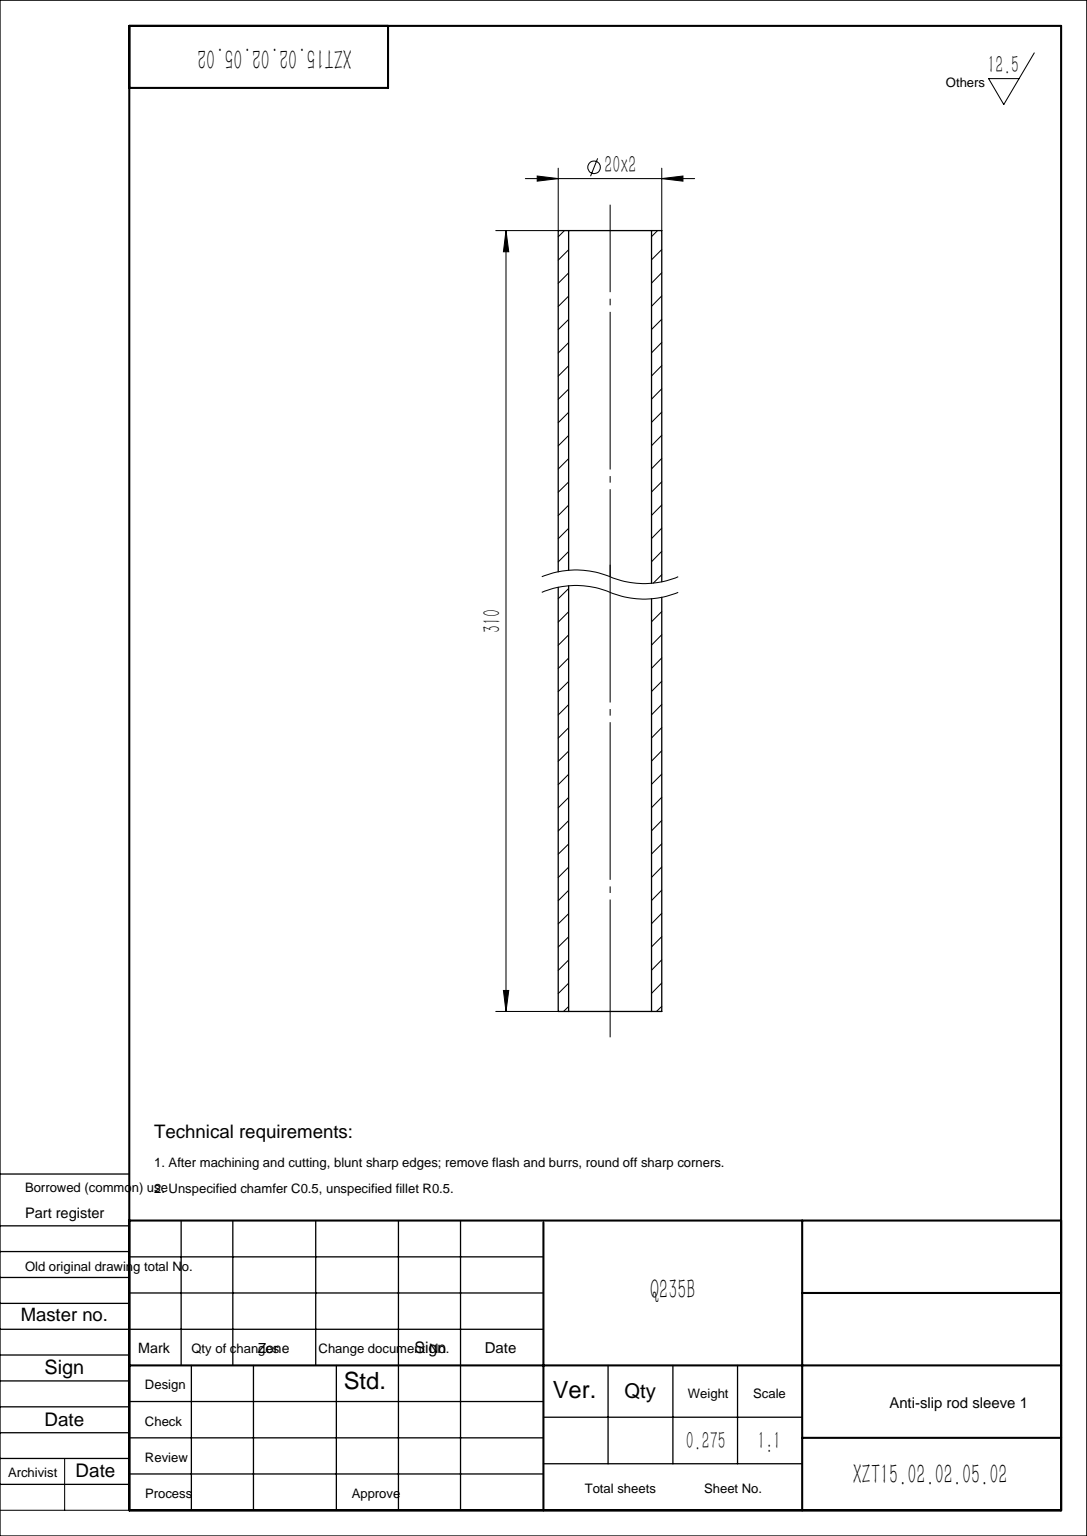
SolidWorks part; units mm, degrees
material "Q235B"
ref_plane "Front Plane" through (0, 0, 0) normal (0, 0, 1) x (1, 0, 0)
ref_plane "Top Plane" through (0, 0, 0) normal (0, 1, 0) x (1, 0, 0)
ref_plane "Right Plane" through (0, 0, 0) normal (1, 0, 0) x (0, 0, -1)
sketch "Sketch1" plane through (0, 0, 0) normal (0, 0, 1) x (1, 0, 0)
  line L0 (0, 0) -> (0, 310)
  dimension "D1" = 310
other "Gb／t 6728—2002 round tube 20 × 2(1)"
ref_plane "Plane1" through (0, 0, 0) normal (0, 1, 0) x (-1, 0, 0)
sketch "Sketch11" plane through (0, 0, 0) normal (0, 1, 0) x (-1, 0, 0)
  circle A0 centre (0, 0) radius 8
  circle A1 centre (0, 0) radius 10
  point P3 (0, 0)
  dimension "Out_dia" = 20
  dimension "D1" = 2
